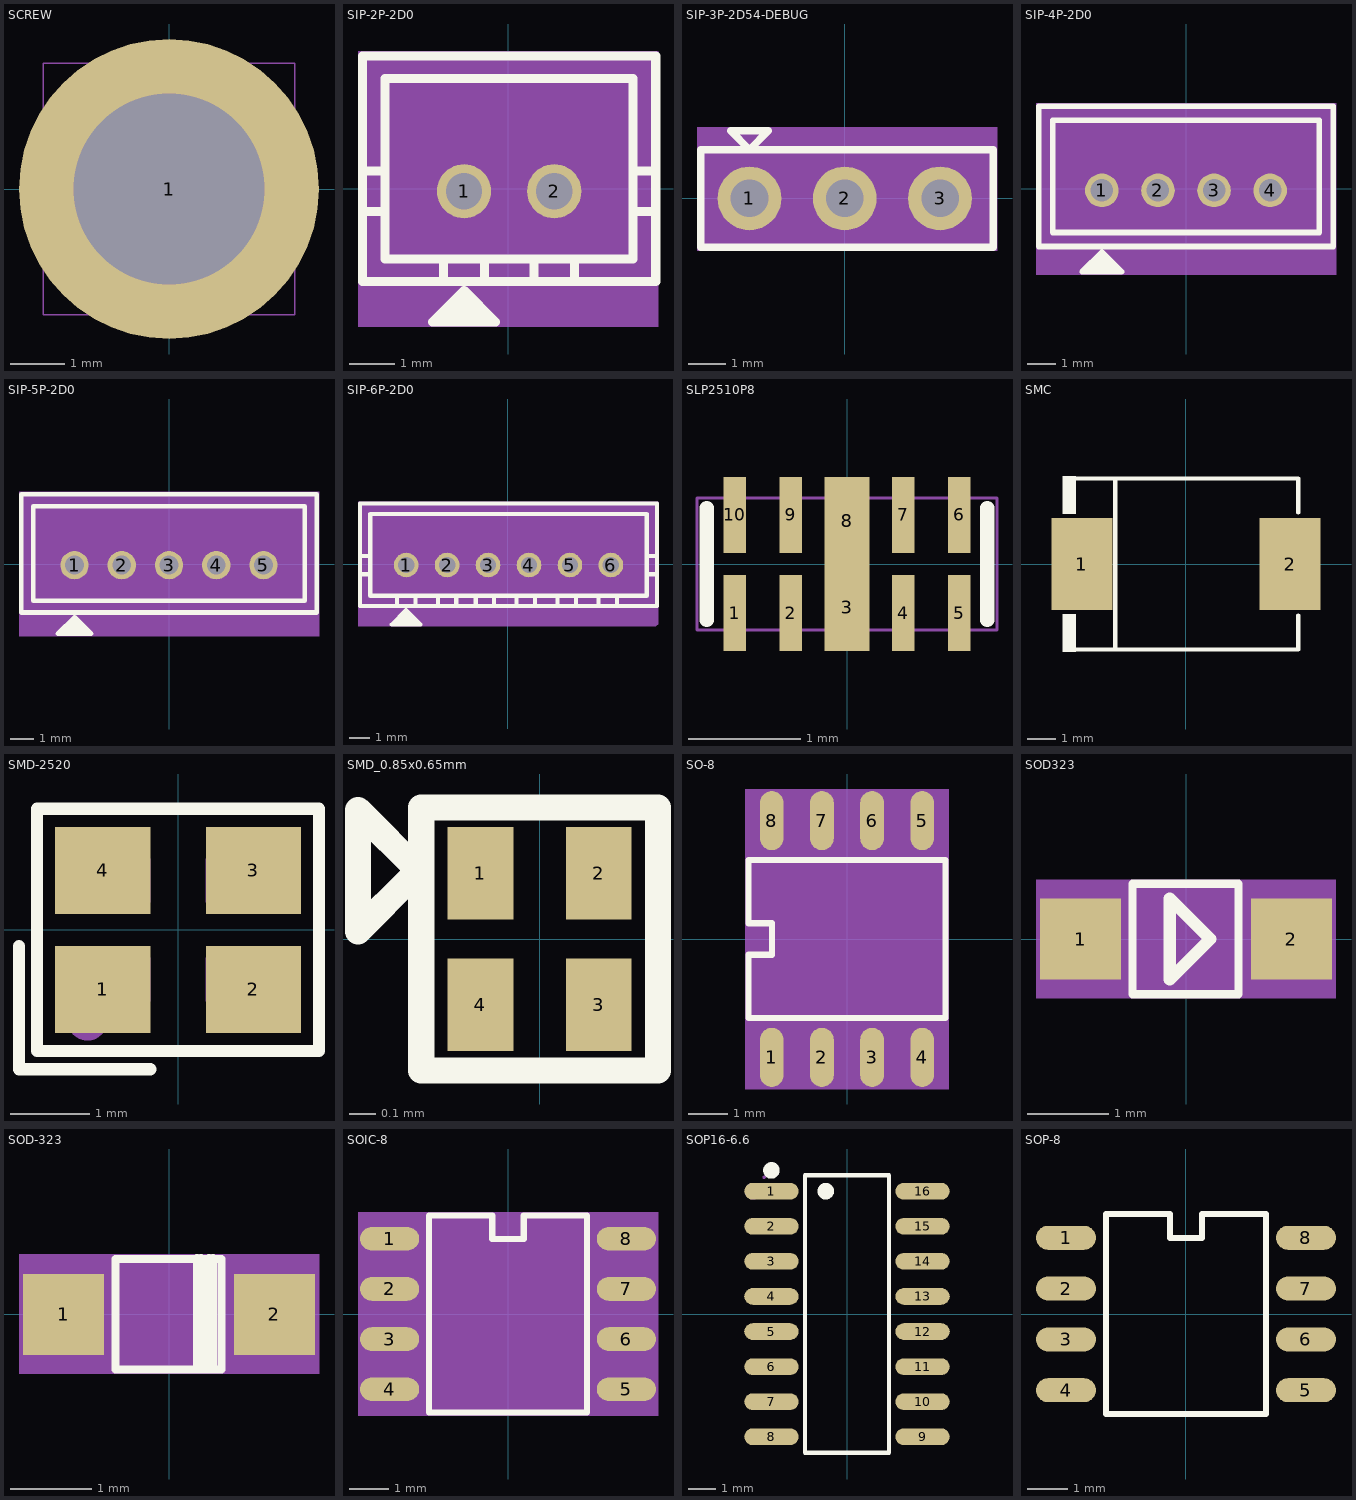
[diagram p0: the footprints below, top view; thin cyan lines are the x and y axes]
# Altium footprint library MISC84456-5.PcbLib: 85 footprints (part 4 of 6)
Each footprint in its own frame and in the unit in brackets; x right, y up, seen from the top. Pads: shape width x height; smd on the part's side, far side on the other; paste and mask are expansions set on the pad; w line width, h text height; cw(c..) or ccw(c..) is an arc to the next point about the centre after c.

## SCREW [mm] "SCREW"
pads (1):
  round 5.5 hole 3.5: 1(0,0)
Mechanical 7:
  text "1" at -0.063,0 h0.08
Mechanical 8:
  lines w0.025: -2.301,-2.301 2.301,-2.301 2.301,2.301 -2.301,2.301 -2.301,-2.301

## SIP-2P-2D0 [mm] "SIP-2P-2D0"
pads (2):
  round 1.2 hole 0.8: 1(-0.975,-0.05) 2(1.025,-0.05)
Top Overlay:
  lines w0.2: -3.225,-0.5 -2.725,-0.5 ; -3.225,0.4 -2.725,0.4 ; -1.425,-2.75 -0.525,-2.75 ; -1.425,-2.05 -1.425,-1.55 ; -1.275,-2.6 -0.675,-2.6 ; -1.125,-2.45 -0.825,-2.45 ; -0.525,-2.05 -0.525,-1.55 ; 0.575,-2.05 0.575,-1.55 ; 1.475,-2.05 1.475,-1.55 ; 2.775,-0.5 3.275,-0.5 ; 2.775,0.4 3.275,0.4 ; -3.225,-2.05 -3.225,2.95 3.275,2.95 3.275,-2.05 -3.225,-2.05 ; -2.725,-1.55 -2.725,2.45 2.775,2.45 2.775,-1.55 -2.725,-1.55 ; -1.675,-2.95 -0.975,-2.25 -0.275,-2.95 -1.675,-2.95
  text ".Designator" at -3.35,-2.6 h0.6
Mechanical 7:
  text "1" at -0.975,0.204 h0.64
  text "2" at 1.025,0.204 h0.64
Mechanical 8:
  region: -3.325,-3.05 3.325,-3.05 3.325,3.05 -3.325,3.05

## SIP-3P-2D54-DEBUG [mm] "SIP-3P-2D54-DEBUG"
pads (3):
  round 1.7 hole 1: 1(-2.54,0) 2(0,0) 3(2.54,0)
Top Overlay:
  lines w0.2: -3.84,0 -3.84,1.3 3.96,1.3 3.96,-1.3 -3.84,-1.3 -3.84,0.1 ; -3.04,1.8 -2.04,1.8 -2.54,1.3 -3.04,1.8
Mechanical 7:
  text "1" at -2.54,-0.254 h0.64
  text "2" at 0,-0.254 h0.64
  text "3" at 2.54,-0.254 h0.64
Mechanical 8:
  region: -3.94,-1.4 4.06,-1.4 4.06,1.9 -3.94,1.9
Mechanical 9:
  text ".Designator" at -1.09,-0.6 h0.35

## SIP-4P-2D0 [mm] "SIP-4P-2D0"
pads (4):
  round 1.2 hole 0.8: 1(-3,-0.05) 2(-1,-0.05) 3(1,-0.05) 4(3,-0.05)
Top Overlay:
  lines w0.2: -3.45,-2.75 -2.55,-2.75 ; -3.3,-2.6 -2.7,-2.6 ; -3.15,-2.45 -2.85,-2.45 ; -5.25,-2.05 -5.25,2.95 3.25,2.95 5.25,2.95 5.25,-2.05 3.25,-2.05 -5.25,-2.05 ; -4.75,-1.55 -4.75,2.45 2.75,2.45 4.75,2.45 4.75,2.05 4.75,-1.55 2.75,-1.55 -4.75,-1.55 ; -3.7,-2.95 -2.3,-2.95 -3,-2.25 -3.7,-2.95
  text ".Designator" at 5.75,0.075 h0.6
Mechanical 7:
  text "4" at 3,0.204 h0.64
  text "3" at 1,0.204 h0.64
  text "2" at -1,0.204 h0.64
  text "1" at -3,0.204 h0.64
Mechanical 8:
  region: -5.35,-3.05 5.35,-3.05 5.35,3.05 -5.35,3.05

## SIP-5P-2D0 [mm] "SIP-5P-2D0"
pads (5):
  round 1.2 hole 0.8: 1(-4,-0.05) 2(-2,-0.05) 3(0,-0.05) 4(2,-0.05) 5(4,-0.05)
Top Overlay:
  lines w0.2: -4.45,-2.75 -3.55,-2.75 ; -4.3,-2.6 -3.7,-2.6 ; -4.15,-2.45 -3.85,-2.45 ; -6.25,-2.05 2.25,-2.05 6.25,-2.05 6.25,2.95 2.25,2.95 -6.25,2.95 -6.25,-2.05 ; -5.75,-1.55 1.75,-1.55 5.75,-1.55 5.75,2.05 5.75,2.45 1.75,2.45 -5.75,2.45 -5.75,-1.55 ; -4.7,-2.95 -4,-2.25 -3.3,-2.95 -4.7,-2.95
Mechanical 7:
  text "3" at 0,0.204 h0.64
  text "2" at -2,0.204 h0.64
  text "1" at -4,0.204 h0.64
  text "5" at 4,0.204 h0.64
  text "4" at 2,0.204 h0.64
Mechanical 8:
  region: -6.35,-3.05 6.35,-3.05 6.35,3.05 -6.35,3.05
Mechanical 9:
  text ".Designator" at 4.625,2.075 h0.35

## SIP-6P-2D0 [mm] "SIP-6P-2D0"
pads (6):
  round 1.2 hole 0.8: 1(-4.975,-0.05) 2(-2.975,-0.05) 3(-0.975,-0.05) 4(1.025,-0.05) 5(3.025,-0.05) 6(5.025,-0.05)
Top Overlay:
  lines w0.2: -7.225,-0.5 -6.725,-0.5 ; -7.225,0.4 -6.725,0.4 ; -5.425,-2.75 -4.525,-2.75 ; -5.425,-2.05 -5.425,-1.55 ; -5.275,-2.6 -4.675,-2.6 ; -5.125,-2.45 -4.825,-2.45 ; -4.525,-2.05 -4.525,-1.55 ; -3.425,-2.05 -3.425,-1.55 ; -2.525,-2.05 -2.525,-1.55 ; -1.575,-2.05 -1.575,-1.55 ; -0.675,-2.05 -0.675,-1.55 ; 0.425,-2.05 0.425,-1.55 ; 1.325,-2.05 1.325,-1.55 ; 2.425,-2.05 2.425,-1.55 ; 3.325,-2.05 3.325,-1.55 ; 4.425,-2.05 4.425,-1.55 ; 5.325,-2.05 5.325,-1.55 ; 6.775,-0.5 7.275,-0.5 ; 6.775,0.4 7.275,0.4 ; -7.225,-2.05 -7.225,2.95 1.275,2.95 5.275,2.95 7.275,2.95 7.275,-2.05 5.275,-2.05 1.275,-2.05 -7.225,-2.05 ; -6.725,-1.55 -6.725,2.45 0.775,2.45 4.775,2.45 6.775,2.45 6.775,-1.55 4.775,-1.55 0.775,-1.55 -6.725,-1.55 ; -5.675,-2.95 -4.275,-2.95 -4.975,-2.25 -5.675,-2.95
  text ".Designator" at -5.525,-2.4 h0.6
Mechanical 7:
  text "2" at -2.721,-0.05 h0.64
  text "5" at 3.279,-0.05 h0.64
  text "6" at 5.279,-0.05 h0.64
  text "1" at -4.721,-0.05 h0.64
  text "4" at 1.279,-0.05 h0.64
  text "3" at -0.721,-0.05 h0.64
Mechanical 8:
  region: -7.325,-3.05 1.375,-3.05 7.225,-3.05 7.325,-2.95 7.325,3.05 1.375,3.05 -7.325,3.05

## SLP2510P8 [mm] "SLP2510P8"
pads (10):
  rect 0.2x0.675 smd: 1(-1,-0.437) 2(-0.5,-0.437) 4(0.5,-0.437) 5(1,-0.437) 6(1,0.437) 7(0.5,0.437) 9(-0.5,0.437) 10(-1,0.437)
  rect 0.4x0.775 smd: 3(0,-0.388) 8(0,0.388)
Top Overlay:
  lines w0.127: -1.25,-0.5 -1.25,0.5 ; 1.25,-0.5 1.25,0.5
  text ".Designator" at -0.625,1.05 h0.6
Mechanical 7:
  text "7" at 0.246,0.437 h0.64
  text "4" at 0.246,-0.437 h0.64
  text "1" at -1.254,-0.437 h0.64
  text "10" at -1.508,0.437 h0.64
  text "6" at 0.746,0.437 h0.64
  text "5" at 0.746,-0.437 h0.64
  text "2" at -0.754,-0.437 h0.64
  text "9" at -0.754,0.437 h0.64
  text "3" at -0.254,-0.388 h0.64
  text "8" at -0.254,0.388 h0.64
Mechanical 8:
  lines w0.025: -1.338,-0.587 1.338,-0.587 1.338,0.588 -1.338,0.588 -1.338,-0.587
Mechanical 9:
  lines w0.025: -1.338,-0.587 1.338,-0.587 1.338,0.588 -1.338,0.588 -1.338,-0.587
  text "TPD4E05U06" at -1.025,-1.45 h0.35

## SMC [mm]
pads (2):
  rect 2.158x3.24 smd: 1(-3.686,0) 2(3.686,0)
Top Overlay:
  region: -3.9,-3.102 -3.9,-1.772 -4.357,-1.772 -4.357,-3.102
  region: -3.9,3.102 -3.9,1.772 -4.357,1.772 -4.357,3.102
  lines w0.152: -3.976,-3.026 3.976,-3.026 3.976,-1.823 ; -3.976,3.026 3.976,3.026 3.976,1.823 ; -2.504,-3.026 -2.504,3.026
Mechanical 5:
  region: -3.95,-1.5 -3.95,1.5 -2.7,1.5 -2.7,-1.5
Mechanical 6:
  circle w0.06: c-4.13,-2.95 r0.03

## SMD-2520 [mm]
pads (4):
  rect 1.2x1.1 smd: 1(-0.95,-0.75) 2(0.95,-0.75) 3(0.95,0.75) 4(-0.95,0.75)
Top Overlay:
  lines w0.152: -2.007,-0.201 -2.007,-1.758 -0.351,-1.758 ; -1.779,-1.529 1.779,-1.529 1.779,1.529 -1.779,1.529 -1.779,-1.529
Mechanical 5:
  region: -1.25,-0.35 -0.35,-0.35 -0.35,-0.9 -1.25,-0.9
  region: 0.35,-0.35 1.25,-0.35 1.25,-0.9 0.35,-0.9
  region: 0.35,0.9 1.25,0.9 1.25,0.35 0.35,0.35
  region: -1.25,0.9 -0.35,0.9 -0.35,0.35 -1.25,0.35
Mechanical 6:
  circle w0.06: c-1.25,-1 r0.03
Mechanical 15:
  circle w0.254: c-1.143,-1.143 r0.127

## SMD_0.85x0.65mm [mm]
pads (4):
  rect 0.25x0.35 smd: 1(-0.225,0.25) 2(0.225,0.25) 3(0.225,-0.25) 4(-0.225,-0.25)
Top Overlay:
  lines w0.1: -0.48,0.24 -0.48,0.24 ; -0.48,0.24 -0.69,0.03 -0.69,0.49 -0.45,0.25 ; -0.45,0.25 -0.45,0.25 ; -0.45,-0.5 0.45,-0.5 0.45,0.5 -0.45,0.5 -0.45,-0.5

## SO-8 [mm] "SO-8"
pads (8):
  oval 0.599x1.501 smd: 1(-1.905,-3) 2(-0.635,-3) 3(0.635,-3) 4(1.905,-3) 5(1.905,3) 6(0.635,3) 7(-0.635,3) 8(-1.905,3)
Top Overlay:
  lines w0.152: -2.499,-1.999 2.499,-1.999 2.499,1.999 -2.499,1.999 -2.499,0.399 -1.9,0.399 -1.9,-0.399 -2.499,-0.399 -2.499,-1.999
  text ".Designator" at 2.9,1.875 h0.6
Mechanical 7:
  text "2" at -0.635,-2.746 h0.64
  text "3" at 0.635,-2.746 h0.64
  text "5" at 1.905,3.254 h0.64
  text "1" at -1.905,-2.746 h0.64
  text "8" at -1.905,3.254 h0.64
  text "4" at 1.905,-2.746 h0.64
  text "7" at -0.635,3.254 h0.64
  text "6" at 0.635,3.254 h0.64
Mechanical 8:
  region: -2.576,-3.8 2.576,-3.8 2.576,3.8 -2.576,3.8
Mechanical 9:
  text "TJA1040T" at 0,1.625 h0.35

## SOD323 [mm] "SOD323"
pads (2):
  rect 1x1 smd: 1(-1.3,0) 2(1.3,0)
Top Overlay:
  lines w0.1: -0.659,-0.681 0.646,-0.681 0.646,0.681 -0.659,0.681 -0.659,-0.681
  lines w0.15: -0.2,-0.5 -0.2,0.5 0.3,0 -0.2,-0.5
Mechanical 7:
  text "2" at 1.3,0.254 h0.64
  text "1" at -1.3,0.254 h0.64
Mechanical 8:
  region: -1.85,-0.731 1.85,-0.731 1.85,0.731 -1.85,0.731
Mechanical 9:
  text ".Designator" at -0.075,0.425 h0.35
  text "B5819WS" at -0.3,1.3 h0.35

## SOD-323 [mm] "SOD-323"
pads (2):
  rect 1.001x1.001 smd: 1(-1.301,-0.005) 2(1.301,-0.005)
Top Overlay:
  lines w0.099: 0.344,-0.683 0.344,0.688 ; 0.394,-0.683 0.394,0.688 ; 0.494,-0.683 0.494,0.688 ; 0.544,-0.683 0.544,0.688 ; -0.658,-0.686 -0.658,0.676 0.645,0.676 0.645,-0.686 -0.658,-0.686
Mechanical 7:
  text "2" at 1.301,0.249 h0.64
  text "1" at -1.301,0.249 h0.64
Mechanical 8:
  region: -1.849,-0.737 1.849,-0.737 1.849,0.737 -1.849,0.737
Mechanical 9:
  text ".Designator" at 0.4,0.22 h0.35
  text "IN4148" at 1.1,0.045 h0.35

## SOIC-8 [mm]
pads (8):
  oval 1.501x0.599 smd: 1(-3,1.905) 2(-3,0.635) 3(-3,-0.635) 4(-3,-1.905) 5(3,-1.905) 6(3,-0.635) 7(3,0.635) 8(3,1.905)
Top Overlay:
  lines w0.152: -1.999,-2.499 1.999,-2.499 1.999,2.499 0.399,2.499 0.399,1.9 -0.399,1.9 -0.399,2.499 -1.999,2.499 -1.999,-2.499
  text ".Designator" at 1.875,-2.9 h0.6
Mechanical 7:
  text "2" at -2.746,0.635 h0.64
  text "3" at -2.746,-0.635 h0.64
  text "5" at 3.254,-1.905 h0.64
  text "1" at -2.746,1.905 h0.64
  text "8" at 3.254,1.905 h0.64
  text "4" at -2.746,-1.905 h0.64
  text "7" at 3.254,0.635 h0.64
  text "6" at 3.254,-0.635 h0.64
Mechanical 8:
  region: -3.8,2.576 -3.8,-2.576 3.8,-2.576 3.8,2.576
Mechanical 9:
  text "TJA1040T" at 1.625,0 h0.35

## SOP16-6.6 [mm]
pads (16):
  oval 1.971x0.602 smd: 1(-2.736,4.445) 2(-2.736,3.175) 3(-2.736,1.905) 4(-2.736,0.635) 5(-2.736,-0.635) 6(-2.736,-1.905) 7(-2.736,-3.175) 8(-2.736,-4.445) 9(2.736,-4.445) 10(2.736,-3.175) 11(2.736,-1.905) 12(2.736,-0.635) 13(2.736,0.635) 14(2.736,1.905) 15(2.736,3.175) 16(2.736,4.445)
Top Overlay:
  circle w0.3: c-0.769,4.445 r0.15
  circle w0.3: c-2.736,5.198 r0.15
  lines w0.152: -1.521,-5.026 1.521,-5.026 1.521,5.026 -1.521,5.026 -1.521,-5.026
Mechanical 5:
  region: -3,4.66 -2.3,4.66 -2.3,4.23 -3,4.23
  pour cut-out: -2.31,4.66 -1.94,4.66 -1.94,4.23 -2.31,4.23
  region: -3,3.39 -2.3,3.39 -2.3,2.96 -3,2.96
  pour cut-out: -2.31,3.39 -1.94,3.39 -1.94,2.96 -2.31,2.96
  region: -3,2.12 -2.3,2.12 -2.3,1.69 -3,1.69
  pour cut-out: -2.31,2.12 -1.94,2.12 -1.94,1.69 -2.31,1.69
  region: -3,0.85 -2.3,0.85 -2.3,0.42 -3,0.42
  pour cut-out: -2.31,0.85 -1.94,0.85 -1.94,0.42 -2.31,0.42
  region: -3,-0.42 -2.3,-0.42 -2.3,-0.85 -3,-0.85
  pour cut-out: -2.31,-0.42 -1.94,-0.42 -1.94,-0.85 -2.31,-0.85
  region: -3,-1.69 -2.3,-1.69 -2.3,-2.12 -3,-2.12
  pour cut-out: -2.31,-1.69 -1.94,-1.69 -1.94,-2.12 -2.31,-2.12
  region: -3,-2.96 -2.3,-2.96 -2.3,-3.39 -3,-3.39
  pour cut-out: -2.31,-2.96 -1.94,-2.96 -1.94,-3.39 -2.31,-3.39
  region: -3,-4.23 -2.3,-4.23 -2.3,-4.66 -3,-4.66
  pour cut-out: -2.31,-4.23 -1.94,-4.23 -1.94,-4.66 -2.31,-4.66
  region: 3,4.66 2.3,4.66 2.3,4.23 3,4.23
  pour cut-out: 2.31,4.66 1.94,4.66 1.94,4.23 2.31,4.23
  region: 3,3.39 2.3,3.39 2.3,2.96 3,2.96
  pour cut-out: 2.31,3.39 1.94,3.39 1.94,2.96 2.31,2.96
  region: 3,2.12 2.3,2.12 2.3,1.69 3,1.69
  pour cut-out: 2.31,2.12 1.94,2.12 1.94,1.69 2.31,1.69
  region: 3,0.85 2.3,0.85 2.3,0.42 3,0.42
  pour cut-out: 2.31,0.85 1.94,0.85 1.94,0.42 2.31,0.42
  region: 3,-0.42 2.3,-0.42 2.3,-0.85 3,-0.85
  pour cut-out: 2.31,-0.42 1.94,-0.42 1.94,-0.85 2.31,-0.85
  region: 3,-1.69 2.3,-1.69 2.3,-2.12 3,-2.12
  pour cut-out: 2.31,-1.69 1.94,-1.69 1.94,-2.12 2.31,-2.12
  region: 3,-2.96 2.3,-2.96 2.3,-3.39 3,-3.39
  pour cut-out: 2.31,-2.96 1.94,-2.96 1.94,-3.39 2.31,-3.39
  region: 3,-4.23 2.3,-4.23 2.3,-4.66 3,-4.66
  pour cut-out: 2.31,-4.23 1.94,-4.23 1.94,-4.66 2.31,-4.66
Mechanical 6:
  circle w0.06: c-3,4.95 r0.03
Mechanical 15:
  circle w0.3: c-3.4,4.445 r0.15

## SOP-8 [mm]
pads (8):
  oval 1.501x0.599 smd: 1(-3,1.905) 2(-3,0.635) 3(-3,-0.635) 4(-3,-1.905) 5(3,-1.905) 6(3,-0.635) 7(3,0.635) 8(3,1.905)
Top Overlay:
  lines w0.152: -1.999,-2.499 1.999,-2.499 1.999,2.499 0.399,2.499 0.399,1.9 -0.399,1.9 -0.399,2.499 -1.999,2.499 -1.999,-2.499
Mechanical 7:
  text "2" at -2.746,0.635 h0.64
  text "3" at -2.746,-0.635 h0.64
  text "5" at 3.254,-1.905 h0.64
  text "1" at -2.746,1.905 h0.64
  text "8" at 3.254,1.905 h0.64
  text "4" at -2.746,-1.905 h0.64
  text "7" at 3.254,0.635 h0.64
  text "6" at 3.254,-0.635 h0.64
Mechanical 9:
  text "TJA1040T" at 1.625,0 h0.35